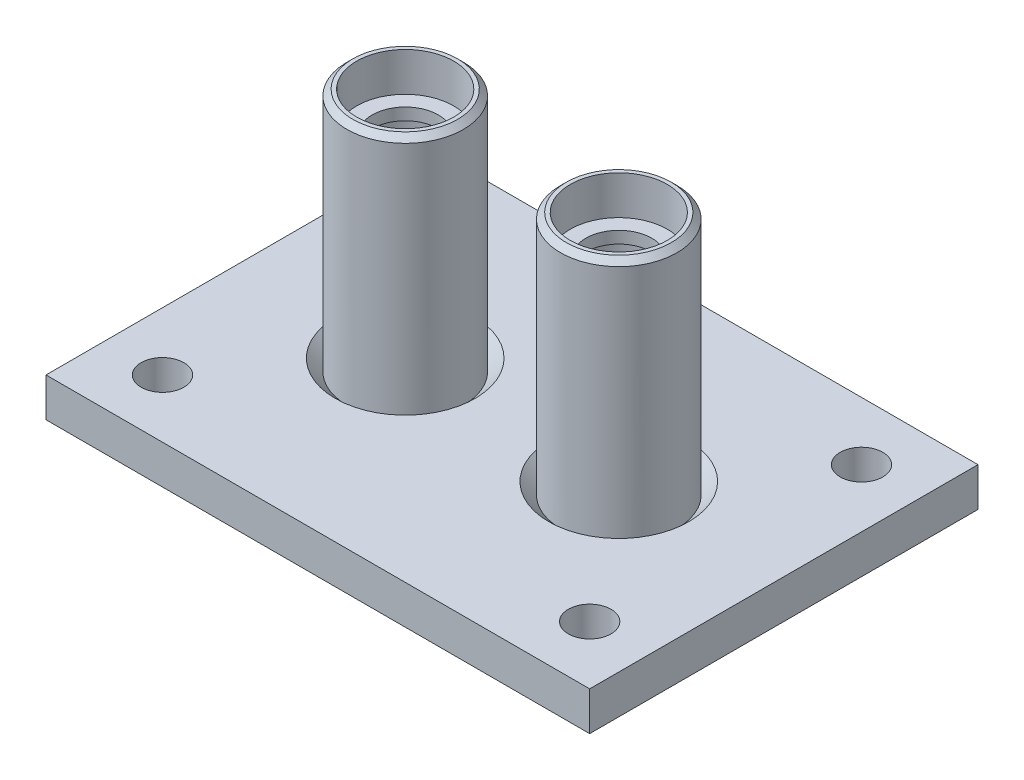
from build123d import *

# Parameters (mm, degrees)
SKETCH_2_7_R        = 11
BOSS_EXTRUDE2_DEPTH = 20
CHAMFER1_SIZE       = 6
SKETCH_2_7_2_R      = 30
BOSS_EXTRUDE5_DEPTH = 140
SKETCH4_R           = 25
CUT_EXTRUDE2_DEPTH  = 20
SKETCH5_R           = 20
CUT_EXTRUDE3_DEPTH  = 112
SKETCH6_R           = 17
CUT_EXTRUDE4_DEPTH  = 8
CHAMFER2_SIZE       = 3
CUT_EXTRUDE5_START  = -112
SKETCH7_R           = 21.25
CUT_EXTRUDE5_DEPTH  = 1.85


with BuildPart() as part:
    # Sketch 2_7 → Boss-Extrude2 (new body)
    # profile 1 of 7: a face of its own
    with BuildSketch(Plane(origin=(0, 0, 0), x_dir=(1, 0, 0), z_dir=(0, 1, 0))):
        Polygon((-140, -100), (-85, -100), (-85, -4.73e-07), (-85, 100), (-140, 100), align=None)
        with Locations(Location((-110, -70, 0), (0, 0, 270))):
            Circle(SKETCH_2_7_R, mode=Mode.SUBTRACT)
        with Locations(Location((-110, 70, 0), (0, 0, 270))):
            Circle(SKETCH_2_7_R, mode=Mode.SUBTRACT)
    # profile 2 of 7: a face of its own
    with BuildSketch(Plane(origin=(0, 0, 0), x_dir=(1, 0, 0), z_dir=(0, 1, 0))):
        with BuildLine():
            Line((-85, -100), (-25, -100))
            Line((-25, -100), (-25, 0))
            ThreePointArc((-25, 0), (-54.999999763, -30), (-85, -4.73e-07))
            Line((-85, -4.73e-07), (-85, -100))
        make_face()
    # profile 3 of 7: a face of its own
    with BuildSketch(Plane(origin=(0, 0, 0), x_dir=(1, 0, 0), z_dir=(0, 1, 0))):
        with BuildLine():
            ThreePointArc((-85, -4.73e-07), (-55.000000237, 30), (-25, 0))
            Line((-25, 0), (-25, 100))
            Line((-25, 100), (-85, 100))
            Line((-85, 100), (-85, -4.73e-07))
        make_face()
    # profile 4 of 7: a face of its own
    with BuildSketch(Plane(origin=(0, 0, 0), x_dir=(1, 0, 0), z_dir=(0, 1, 0))):
        Polygon((-25, -100), (25, -100), (25, 5.4e-08), (25, 100), (-25, 100), (-25, 0), align=None)
    # profile 5 of 7: a face of its own
    with BuildSketch(Plane(origin=(0, 0, 0), x_dir=(1, 0, 0), z_dir=(0, 1, 0))):
        Polygon((85, -100), (140, -100), (140, 100), (85, 100), (85, 0), align=None)
        with Locations(Location((110, -70, 0), (0, 0, 270))):
            Circle(SKETCH_2_7_R, mode=Mode.SUBTRACT)
        with Locations(Location((110, 70, 0), (0, 0, 270))):
            Circle(SKETCH_2_7_R, mode=Mode.SUBTRACT)
    # profile 6 of 7: a face of its own
    with BuildSketch(Plane(origin=(0, 0, 0), x_dir=(1, 0, 0), z_dir=(0, 1, 0))):
        with BuildLine():
            ThreePointArc((25, 5.4e-08), (55.000000027, 30), (85, 0))
            Line((85, 0), (85, 100))
            Line((85, 100), (25, 100))
            Line((25, 100), (25, 5.4e-08))
        make_face()
    # profile 7 of 7: a face of its own
    with BuildSketch(Plane(origin=(0, 0, 0), x_dir=(1, 0, 0), z_dir=(0, 1, 0))):
        with BuildLine():
            Line((25, -100), (85, -100))
            Line((85, -100), (85, 0))
            ThreePointArc((85, 0), (54.999999973, -30), (25, 5.4e-08))
            Line((25, 5.4e-08), (25, -100))
        make_face()
    extrude(amount=BOSS_EXTRUDE2_DEPTH)

    # Chamfer1
    chamfer1_edges = [part.edges().sort_by_distance(p)[0] for p in [
        (-85, 0, 0),
        (85, 0, 5.4e-08),
        (85, 20, 5.4e-08),
        (-85, 20, 0),
    ]]
    chamfer(chamfer1_edges, length=CHAMFER1_SIZE)


with BuildPart() as body_2:
    # Sketch 2_7 2 → Boss-Extrude5 (new body)
    with BuildSketch(Plane(origin=(0, 0, 0), x_dir=(1, 0, 0), z_dir=(0, 1, 0))):
        with Locations(Location((-55, 0, 0), (0, 0, 270))):
            Circle(SKETCH_2_7_2_R)
    extrude(amount=BOSS_EXTRUDE5_DEPTH)

    # Sketch4 → Cut-Extrude2 (cut)
    with BuildSketch(Plane(origin=(0, 140, 0), x_dir=(1, 0, 0), z_dir=(0, 1, 0))):
        with Locations(Location((-55, 0, 0), (0, 0, 270))):
            Circle(SKETCH4_R)
    extrude(amount=-CUT_EXTRUDE2_DEPTH, mode=Mode.SUBTRACT)

    # Sketch5 → Cut-Extrude3 (cut)
    with BuildSketch(Plane.XZ):
        with Locations(Location((-55, 0, 0), (0, 0, 270))):
            Circle(SKETCH5_R)
    extrude(amount=-CUT_EXTRUDE3_DEPTH, mode=Mode.SUBTRACT)

    # Sketch6 → Cut-Extrude4 (cut)
    with BuildSketch(Plane(origin=(0, 120, 0), x_dir=(1, 0, 0), z_dir=(0, 1, 0))):
        with Locations(Location((-55, 0, 0), (0, 0, 270))):
            Circle(SKETCH6_R)
    extrude(amount=-CUT_EXTRUDE4_DEPTH, mode=Mode.SUBTRACT)

    # Chamfer2
    chamfer2_edges = [body_2.edges().sort_by_distance(p)[0] for p in [
        (-55, 140, -30),
    ]]
    chamfer(chamfer2_edges, length=CHAMFER2_SIZE)


with BuildPart() as body_3:
    # Mirror1: mirrored copy
    add(body_2.part.mirror(Plane(origin=(0, 0, 0), x_dir=(0, 0, 1), z_dir=(1, 0, 0))))


with BuildPart() as cut_extrude5_tool:
    # Sketch7 → Cut-Extrude5 (new body)
    with BuildSketch(Plane.XZ.offset(CUT_EXTRUDE5_START)):
        with Locations(Location((-55, 0, 0), (0, 0, 270))):
            Circle(SKETCH7_R)
        with Locations(Location((55, 0, 0), (0, 0, 90))):
            Circle(SKETCH7_R)
    extrude(amount=-CUT_EXTRUDE5_DEPTH)


with BuildPart() as body_2_1:
    add(body_2.part)

    # Cut-Extrude5: cut by cut_extrude5_tool
    add(cut_extrude5_tool.part, mode=Mode.SUBTRACT)


with BuildPart() as body_3_1:
    add(body_3.part)

    # Cut-Extrude5: cut by cut_extrude5_tool
    add(cut_extrude5_tool.part, mode=Mode.SUBTRACT)


solid = Compound([part.part, body_2_1.part, body_3_1.part])
